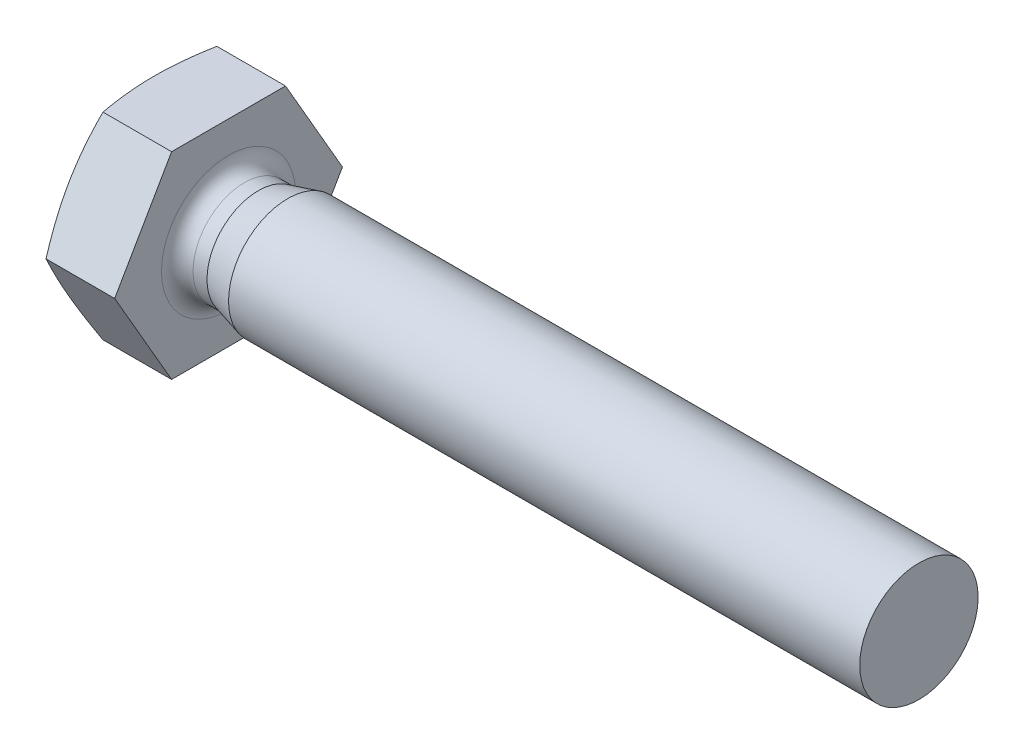
from build123d import *

# Parameters (mm, degrees)
BASEHEAD_DEPTH     = 4
SKETCH6_R          = 4.35
CUT_EXTRUDE1_DEPTH = 1.4
CUT_EXTRUDE2_DEPTH = 0.572
CIRPATTERN2_COUNT  = 2
CIRPATTERN2_ANGLE  = 90


with BuildPart() as part:
    # Sketch2 → BaseHead (new body)
    with BuildSketch(Plane(origin=(0, 0, 0), x_dir=(0, 0, -1), z_dir=(1, 0, 0))):
        Polygon((2.886751346, -5), (5.773502692, 0), (2.886751346, 5), (-2.886751346, 5), (-5.773502692, 0), (-2.886751346, -5), align=None)
    extrude(amount=BASEHEAD_DEPTH)

    # Sketch10 → Revolve1 (revolve)
    with BuildSketch(Plane(origin=(0, 0, 0), x_dir=(1, 0, 0), z_dir=(0, 1, 0)), mode=Mode.PRIVATE) as revolve1_sk:
        with BuildLine():
            Line((4, 3.4), (4, 0))
            Line((4, 0), (39, 0))
            Line((39, 0), (39, 3))
            Line((39, 3), (7, 3))
            Line((7, 3), (5.507179677, 2.6))
            Line((5.507179677, 2.6), (4.8, 2.6))
            ThreePointArc((4.8, 2.6), (4.234314575, 2.834314575), (4, 3.4))
        make_face()
    revolve(revolve1_sk.sketch.rotate(Axis((0, 0, 0), (1, 0, 0)), 180), axis=Axis((0, 0, 0), (1, 0, 0)))

    # Sketch5 → HeadChamfer (revolve, cut)
    with BuildSketch(Plane(origin=(0, 0, 0), x_dir=(1, 0, 0), z_dir=(0, 1, 0)), mode=Mode.PRIVATE) as headchamfer_sk:
        Polygon((0, 5.773502692), (0.518112608, 5.773502692), (0, 4.35), align=None)
    revolve(headchamfer_sk.sketch.rotate(Axis((-0.358389262, 0, 0), (1, 0, 0)), 180), axis=Axis((-0.358389262, 0, 0), (1, 0, 0)), mode=Mode.SUBTRACT)

    # Sketch6 → Cut-Extrude1 (cut)
    with BuildSketch(Plane.ZY):
        Circle(SKETCH6_R)
    extrude(amount=-CUT_EXTRUDE1_DEPTH, mode=Mode.SUBTRACT)

    # Sketch7 → Cut-Extrude2 (cut, symmetric)
    with BuildSketch(Plane(origin=(0, 0, 0), x_dir=(1, 0, 0), z_dir=(0, 1, 0))):
        Polygon((4.26, 0), (0.9, 3.641958042), (0.9, -3.641958042), align=None)
    cut_extrude2 = extrude(amount=CUT_EXTRUDE2_DEPTH, both=True, mode=Mode.SUBTRACT)

    # CirPattern2: Cut-Extrude2 ×2 about axis
    cirpattern2_axis = Axis((0, 0, 0), (-1, 0, 0))
    for i in range(1, CIRPATTERN2_COUNT):
        add(cut_extrude2.rotate(cirpattern2_axis, i * CIRPATTERN2_ANGLE / (CIRPATTERN2_COUNT - 1)), mode=Mode.SUBTRACT)


solid = part.part
